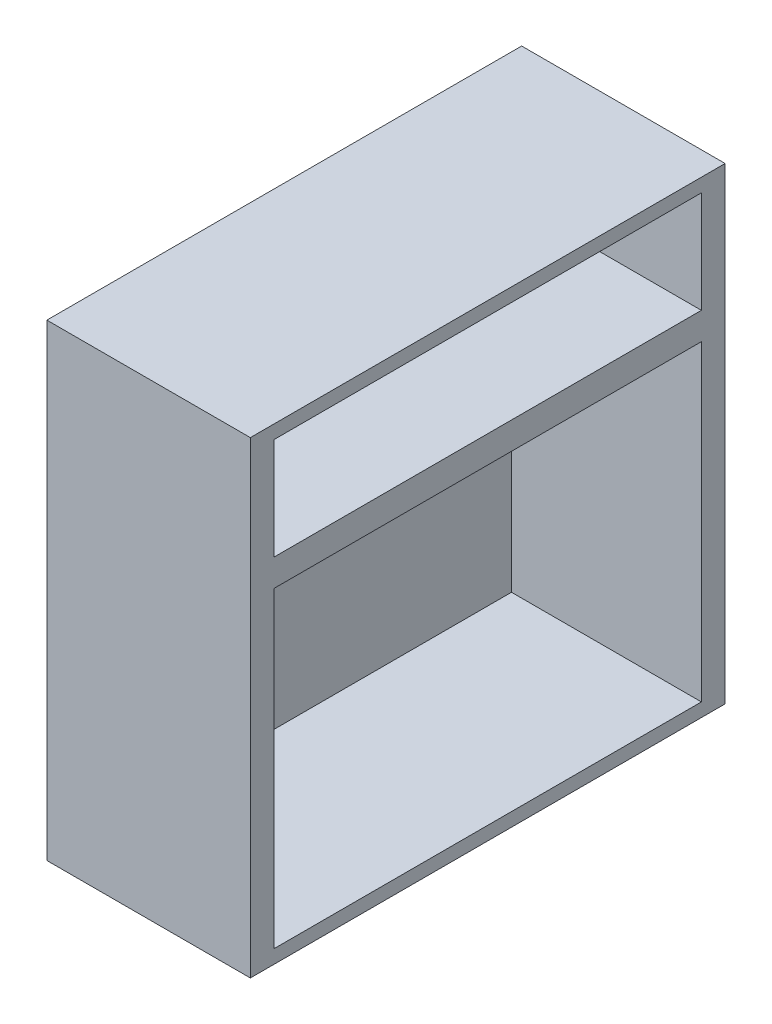
from build123d import *

# Parameters (mm, degrees)
SKETCH1_W           = 300
SKETCH1_H           = 690
BOSS_EXTRUDE1_DEPTH = 700
SKETCH2_W           = 630
SKETCH2_H           = 150
CUT_EXTRUDE1_DEPTH  = 280
SKETCH3_W           = 630
SKETCH3_H           = 460
CUT_EXTRUDE2_DEPTH  = 280


with BuildPart() as part:
    # Sketch1 → Boss-Extrude1 (new body)
    with BuildSketch(Plane.XY):
        Rectangle(SKETCH1_W, SKETCH1_H)
    extrude(amount=BOSS_EXTRUDE1_DEPTH)

    # Sketch2 → Cut-Extrude1 (cut)
    with BuildSketch(Plane(origin=(150, 0, 0), x_dir=(0, 0, -1), z_dir=(1, 0, 0))):
        with Locations((-350, 250)):
            Rectangle(SKETCH2_W, SKETCH2_H)
    extrude(amount=-CUT_EXTRUDE1_DEPTH, mode=Mode.SUBTRACT)

    # Sketch3 → Cut-Extrude2 (cut)
    with BuildSketch(Plane(origin=(150, 0, 0), x_dir=(0, 0, -1), z_dir=(1, 0, 0))):
        with Locations((-350, -95)):
            Rectangle(SKETCH3_W, SKETCH3_H)
    extrude(amount=-CUT_EXTRUDE2_DEPTH, mode=Mode.SUBTRACT)


solid = part.part
